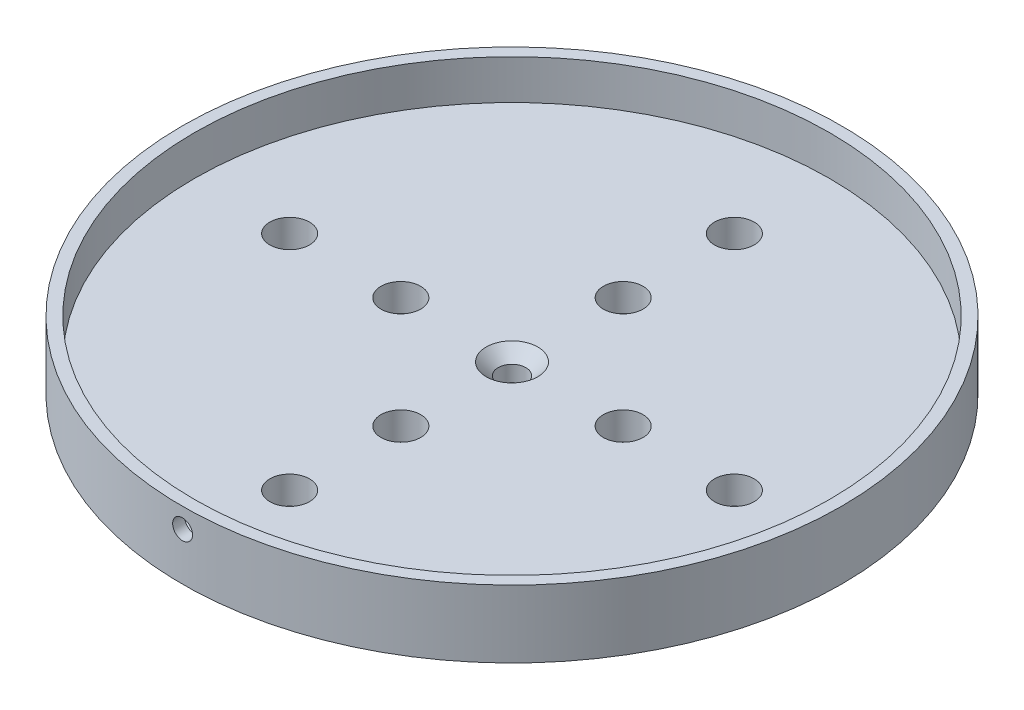
from build123d import *

# Parameters (mm, degrees)
CUT_EXTRUDE1_REACH     = 60.902
SKETCH2_R              = 2.5
M3_TAPPED_HOLE1_REACH  = 94.991
M3_TAPPED_HOLE1_BORE_R = 1.25


with BuildPart() as part:
    # Sketch1 → Revolve1 (revolve)
    with BuildSketch(Plane.XY, mode=Mode.PRIVATE) as revolve1_sk:
        Polygon((1.75, 0), (1.75, 2), (3.25, 3.5), (40, 3.5), (40, 8.5), (41.5, 8.5), (41.5, 0), align=None)
    revolve(revolve1_sk.sketch.rotate(Axis((0, 9.310126582, 0), (0, -1, 0)), 180), axis=Axis((0, 9.310126582, 0), (0, -1, 0)))

    # Sketch2 → Cut-Extrude1 (cut, up to next)
    with BuildSketch(Plane(origin=(0, 3.5, 0), x_dir=(1, 0, 0), z_dir=(0, 1, 0)), mode=Mode.PRIVATE) as cut_extrude1_sk1:
        with Locations(Location((0, 14, 0), (0, 0, 180))):
            Circle(SKETCH2_R)
    cut_extrude1_tool1 = extrude(cut_extrude1_sk1.sketch, amount=-CUT_EXTRUDE1_REACH, mode=Mode.PRIVATE) & part.part
    # Sketch2 → Cut-Extrude1 (cut, up to next)
    with BuildSketch(Plane(origin=(0, 3.5, 0), x_dir=(1, 0, 0), z_dir=(0, 1, 0)), mode=Mode.PRIVATE) as cut_extrude1_sk2:
        with Locations(Location((14, 0, 0), (0, 0, 180))):
            Circle(SKETCH2_R)
    cut_extrude1_tool2 = extrude(cut_extrude1_sk2.sketch, amount=-CUT_EXTRUDE1_REACH, mode=Mode.PRIVATE) & part.part
    # Sketch2 → Cut-Extrude1 (cut, up to next)
    with BuildSketch(Plane(origin=(0, 3.5, 0), x_dir=(1, 0, 0), z_dir=(0, 1, 0)), mode=Mode.PRIVATE) as cut_extrude1_sk3:
        with Locations(Location((0, 28, 0), (0, 0, 180))):
            Circle(SKETCH2_R)
    cut_extrude1_tool3 = extrude(cut_extrude1_sk3.sketch, amount=-CUT_EXTRUDE1_REACH, mode=Mode.PRIVATE) & part.part
    # Sketch2 → Cut-Extrude1 (cut, up to next)
    with BuildSketch(Plane(origin=(0, 3.5, 0), x_dir=(1, 0, 0), z_dir=(0, 1, 0)), mode=Mode.PRIVATE) as cut_extrude1_sk4:
        with Locations(Location((28, 0, 0), (0, 0, 180))):
            Circle(SKETCH2_R)
    cut_extrude1_tool4 = extrude(cut_extrude1_sk4.sketch, amount=-CUT_EXTRUDE1_REACH, mode=Mode.PRIVATE) & part.part
    # Sketch2 → Cut-Extrude1 (cut, up to next)
    with BuildSketch(Plane(origin=(0, 3.5, 0), x_dir=(1, 0, 0), z_dir=(0, 1, 0)), mode=Mode.PRIVATE) as cut_extrude1_sk5:
        with Locations(Location((0, -14, 0), (0, 0, 180))):
            Circle(SKETCH2_R)
    cut_extrude1_tool5 = extrude(cut_extrude1_sk5.sketch, amount=-CUT_EXTRUDE1_REACH, mode=Mode.PRIVATE) & part.part
    # Sketch2 → Cut-Extrude1 (cut, up to next)
    with BuildSketch(Plane(origin=(0, 3.5, 0), x_dir=(1, 0, 0), z_dir=(0, 1, 0)), mode=Mode.PRIVATE) as cut_extrude1_sk6:
        with Locations(Location((0, -28, 0), (0, 0, 180))):
            Circle(SKETCH2_R)
    cut_extrude1_tool6 = extrude(cut_extrude1_sk6.sketch, amount=-CUT_EXTRUDE1_REACH, mode=Mode.PRIVATE) & part.part
    # Sketch2 → Cut-Extrude1 (cut, up to next)
    with BuildSketch(Plane(origin=(0, 3.5, 0), x_dir=(1, 0, 0), z_dir=(0, 1, 0)), mode=Mode.PRIVATE) as cut_extrude1_sk7:
        with Locations(Location((-14, 0, 0), (0, 0, 180))):
            Circle(SKETCH2_R)
    cut_extrude1_tool7 = extrude(cut_extrude1_sk7.sketch, amount=-CUT_EXTRUDE1_REACH, mode=Mode.PRIVATE) & part.part
    # Sketch2 → Cut-Extrude1 (cut, up to next)
    with BuildSketch(Plane(origin=(0, 3.5, 0), x_dir=(1, 0, 0), z_dir=(0, 1, 0)), mode=Mode.PRIVATE) as cut_extrude1_sk8:
        with Locations(Location((-28, 0, 0), (0, 0, 180))):
            Circle(SKETCH2_R)
    cut_extrude1_tool8 = extrude(cut_extrude1_sk8.sketch, amount=-CUT_EXTRUDE1_REACH, mode=Mode.PRIVATE) & part.part
    add(cut_extrude1_tool1.solids().sort_by_distance((0, 3.5, -14))[0], mode=Mode.SUBTRACT)
    add(cut_extrude1_tool2.solids().sort_by_distance((14, 3.5, 0))[0], mode=Mode.SUBTRACT)
    add(cut_extrude1_tool3.solids().sort_by_distance((0, 3.5, -28))[0], mode=Mode.SUBTRACT)
    add(cut_extrude1_tool4.solids().sort_by_distance((28, 3.5, 0))[0], mode=Mode.SUBTRACT)
    add(cut_extrude1_tool5.solids().sort_by_distance((0, 3.5, 14))[0], mode=Mode.SUBTRACT)
    add(cut_extrude1_tool6.solids().sort_by_distance((0, 3.5, 28))[0], mode=Mode.SUBTRACT)
    add(cut_extrude1_tool7.solids().sort_by_distance((-14, 3.5, 0))[0], mode=Mode.SUBTRACT)
    add(cut_extrude1_tool8.solids().sort_by_distance((-28, 3.5, 0))[0], mode=Mode.SUBTRACT)

    # M3 Tapped Hole1 bore (on position points) → M3 Tapped Hole1 (cut, up to next)
    with BuildSketch(Plane(origin=(0, 6, 41.5), x_dir=(1, 0, 0), z_dir=(0, 0, 1)), mode=Mode.PRIVATE) as m3_tapped_hole1_sk1:
        Circle(M3_TAPPED_HOLE1_BORE_R)
    m3_tapped_hole1_tool1 = extrude(m3_tapped_hole1_sk1.sketch, amount=-M3_TAPPED_HOLE1_REACH, mode=Mode.PRIVATE) & part.part
    add(m3_tapped_hole1_tool1.solids().sort_by_distance((0, 6, 41.5))[0], mode=Mode.SUBTRACT)


solid = part.part
